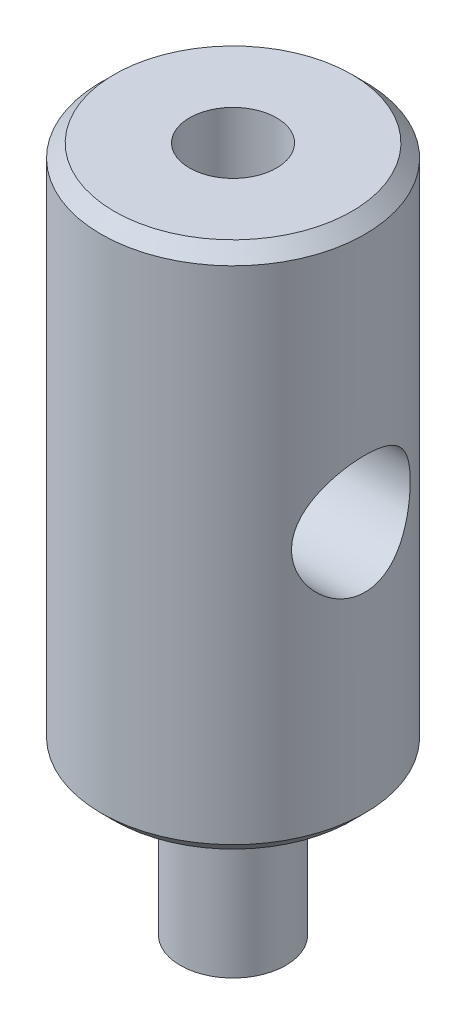
from build123d import *

# Parameters (mm, degrees)
SKETCH1_R               = 5
BOSS_EXTRUDE1_DEPTH     = 10
SKETCH2_R               = 2
BOSS_EXTRUDE2_DEPTH     = 6
SKETCH3_W               = 0.3
SKETCH3_H               = 0.5
M4_TAPPED_HOLE1_D       = 3.3
M4_TAPPED_HOLE1_DEPTH   = 10.1
M4_TAPPED_HOLE1_TIP     = 0.991420021
CHAMFER1_SIZE           = 0.5
CUT_EXTRUDE1_DEPTH      = 18.492855685
CUT_EXTRUDE1_DEPTH_BACK = 18.492855685
SKETCH6_R               = 2.25


with BuildPart() as part:
    # Sketch1 → Boss-Extrude1 (new, symmetric)
    with BuildSketch(Plane(origin=(0, 0, 0), x_dir=(1, 0, 0), z_dir=(0, 1, 0))):
        with Locations(Location((0, 0, 0), (0, 0, 270))):
            Circle(SKETCH1_R)
    extrude(amount=BOSS_EXTRUDE1_DEPTH, both=True)

    # Sketch2 → Boss-Extrude2 (add)
    with BuildSketch(Plane.XZ.offset(10)):
        with Locations(Location((0, 0, 0), (0, 0, 90))):
            Circle(SKETCH2_R)
    extrude(amount=BOSS_EXTRUDE2_DEPTH)

    # Sketch3 → Cut-Revolve1 (revolve, cut)
    with BuildSketch(Plane.XY, mode=Mode.PRIVATE) as cut_revolve1_sk:
        with Locations((1.85, -10.25)):
            Rectangle(SKETCH3_W, SKETCH3_H)
    revolve(cut_revolve1_sk.sketch.rotate(Axis((0, 0, 0), (0, -1, 0)), 90), axis=Axis((0, 0, 0), (0, -1, 0)), mode=Mode.SUBTRACT)

    # M4 Tapped Hole1
    with Locations(Plane(origin=(0, 10, 0), x_dir=(1, 0, 0), z_dir=(0, 1, 0))):
        with Locations((0, 0)):
            Hole(M4_TAPPED_HOLE1_D / 2, depth=M4_TAPPED_HOLE1_DEPTH)
            with Locations((0, 0, -(M4_TAPPED_HOLE1_DEPTH + M4_TAPPED_HOLE1_TIP / 2))):  # 118° drill point
                Cone(0, M4_TAPPED_HOLE1_D / 2, M4_TAPPED_HOLE1_TIP, mode=Mode.SUBTRACT)

    # Chamfer1
    chamfer1_edges = [part.edges().sort_by_distance(p)[0] for p in [
        (0, -10, -5),
        (0, 10, -5),
    ]]
    chamfer(chamfer1_edges, length=CHAMFER1_SIZE)

    # Sketch6 → Cut-Extrude1 (cut, two sides: drawn at the far end of the back side and taken through both)
    with BuildSketch(Plane(origin=(0, 0, 0), x_dir=(0, 0, -1), z_dir=(1, 0, 0)).offset(-CUT_EXTRUDE1_DEPTH_BACK)):
        Circle(SKETCH6_R)
    extrude(amount=CUT_EXTRUDE1_DEPTH + CUT_EXTRUDE1_DEPTH_BACK, mode=Mode.SUBTRACT)


solid = part.part
